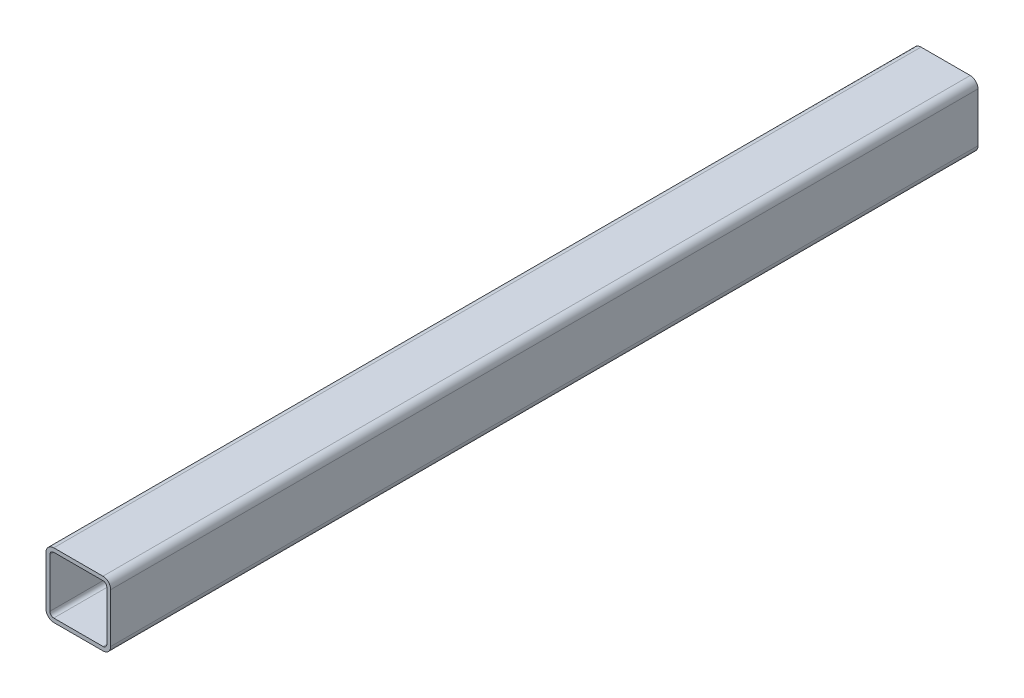
SolidWorks part; units mm, degrees
material "Q235B"
ref_plane "前视基准面" through (0, 0, 0) normal (0, 0, 1) x (1, 0, 0)
ref_plane "上视基准面" through (0, 0, 0) normal (0, 1, 0) x (1, 0, 0)
ref_plane "右视基准面" through (0, 0, 0) normal (1, 0, 0) x (0, 0, -1)
other "Configuration Table"
sketch "草图1" plane through (0, 0, 0) normal (1, 0, 0) x (0, 0, -1)
  line L0 (-335, 0) -> (335, 0)
other "Gb／6728-1986方形空心型钢 050 X 50 X 3(1)"
ref_plane "基准面1" through (0, 0, 335) normal (0, 0, -1) x (0, 1, 0)
sketch "Sketch1" plane through (0, 0, 335) normal (0, 0, -1) x (0, 1, 0)
  line L0 (-19, -22) -> (19, -22)
  line L1 (-22, -19) -> (-22, 19)
  line L2 (19, 22) -> (-19, 22)
  line L3 (22, 19) -> (22, -19)
  line L4 (-19, -25) -> (19, -25)
  line L5 (-25, -19) -> (-25, 19)
  line L6 (19, 25) -> (-19, 25)
  line L7 (25, 19) -> (25, -19)
  arc A0 (25, 19) -> (19, 25) centre (19, 19) ccw
  arc A1 (19, -25) -> (25, -19) centre (19, -19) ccw
  arc A2 (-25, -19) -> (-19, -25) centre (-19, -19) ccw
  arc A3 (-19, 25) -> (-25, 19) centre (-19, 19) ccw
  arc A4 (-19, 22) -> (-22, 19) centre (-19, 19) ccw
  arc A5 (22, 19) -> (19, 22) centre (19, 19) ccw
  arc A6 (19, -22) -> (22, -19) centre (19, -19) ccw
  arc A7 (-22, -19) -> (-19, -22) centre (-19, -19) ccw
  point P0 (-25, 0)
  point P1 (25, 0)
  point P2 (0, 25)
  point P3 (0, -25)
  point P4 (0, 0)
  point P5 (-25, -25)
  point P6 (25, -25)
  point P7 (25, 25)
  point P8 (-25, 25)
  point P33 (0, 0)
  dimension "D1" = 6
  dimension "Thickness" = 3
  dimension "V_leg" = 50
equation "\"D2@草图1\"=\"D1@草图1\"/2"
